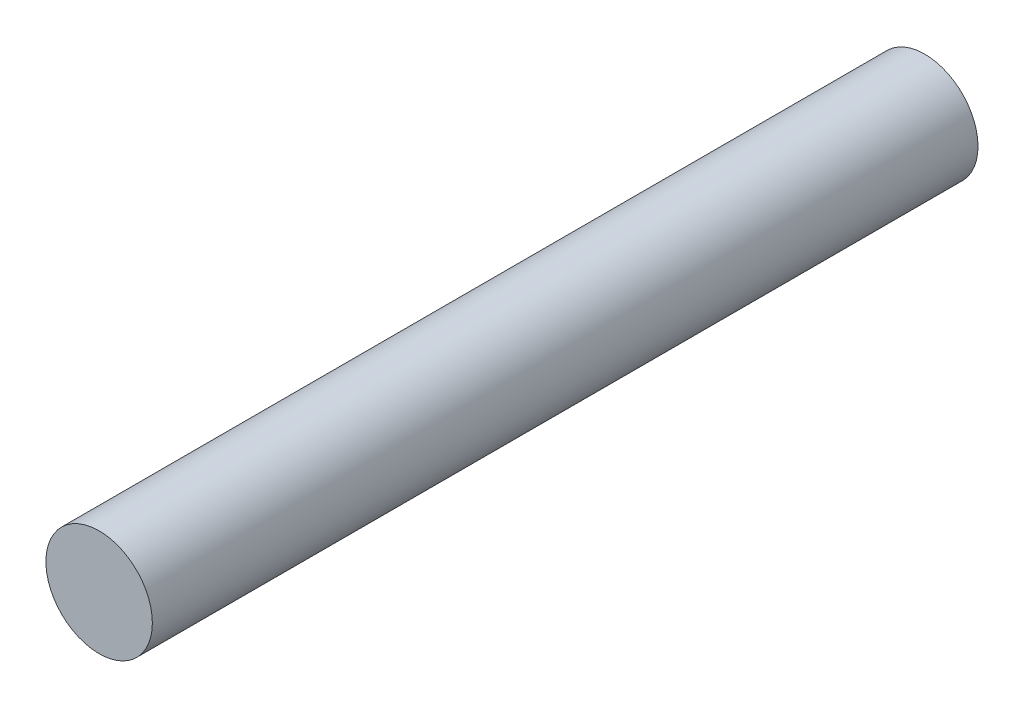
SolidWorks part; units mm, degrees
ref_plane "前视基准面" through (0, 0, 0) normal (0, 0, 1) x (1, 0, 0)
ref_plane "上视基准面" through (0, 0, 0) normal (0, 1, 0) x (1, 0, 0)
ref_plane "右视基准面" through (0, 0, 0) normal (1, 0, 0) x (0, 0, -1)
sketch "草图1" plane through (0, 0, 0) normal (0, 0, 1) x (1, 0, 0)
  circle A0 centre (0, 0) radius 2.45
  dimension "D1" = 4.9
extrude "凸台-拉伸1" add sketch "草图1" along normal blind 38
